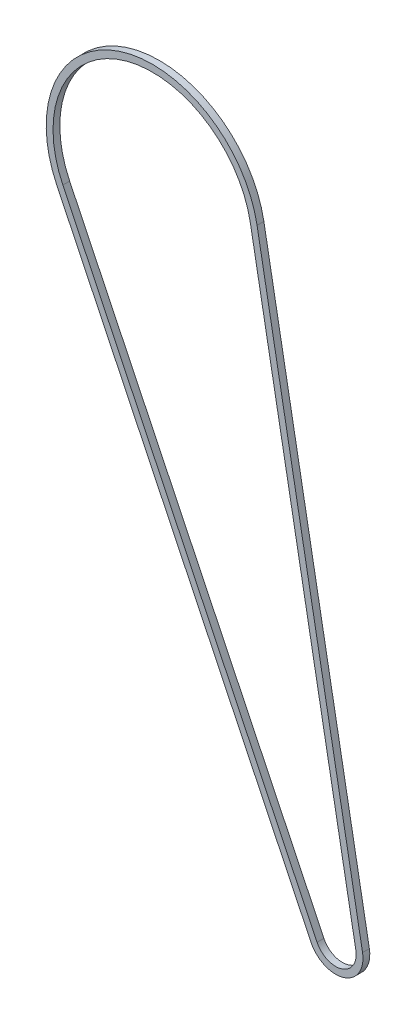
SolidWorks part; units mm, degrees
ref_plane "Front Plane" through (0, 0, 0) normal (0, 0, 1) x (1, 0, 0)
ref_plane "Top Plane" through (0, 0, 0) normal (0, 1, 0) x (1, 0, 0)
ref_plane "Right Plane" through (0, 0, 0) normal (1, 0, 0) x (0, 0, -1)
sketch "Sketch1" plane through (0, 0, 0) normal (0, 0, 1) x (1, 0, 0)
  line L2 (143.673, 109.8712) -> (298.5468, -737.354)
  line L3 (-131.6244, 20.3089) -> (241.6417, -755.8669)
  arc A7 (241.6417, -755.8669) -> (298.5468, -737.354) centre (268.849, -742.7828) ccw
  arc A8 (143.673, 109.8712) -> (-131.6244, 20.3089) centre (0, 83.6076) ccw
extrude "Thin-wall extrude1" add sketch "Sketch1" along normal blind 10 thin thin type one direction wall 10
